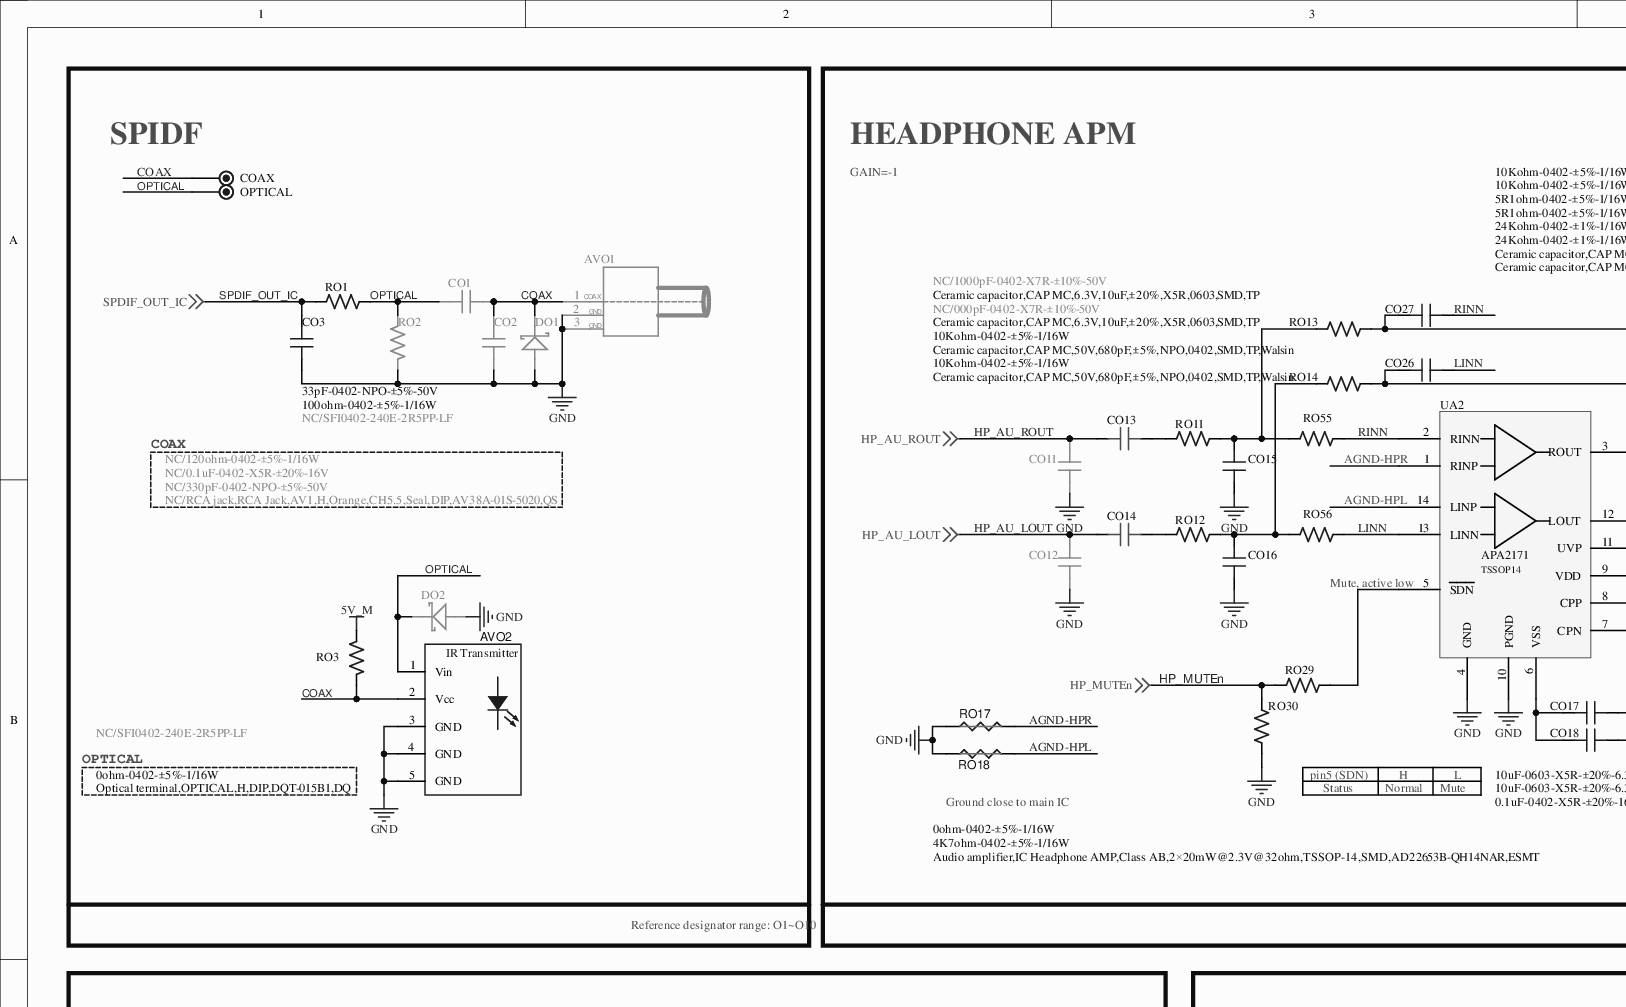
[diagram p0: MISC86290-14.SchDoc, top left]
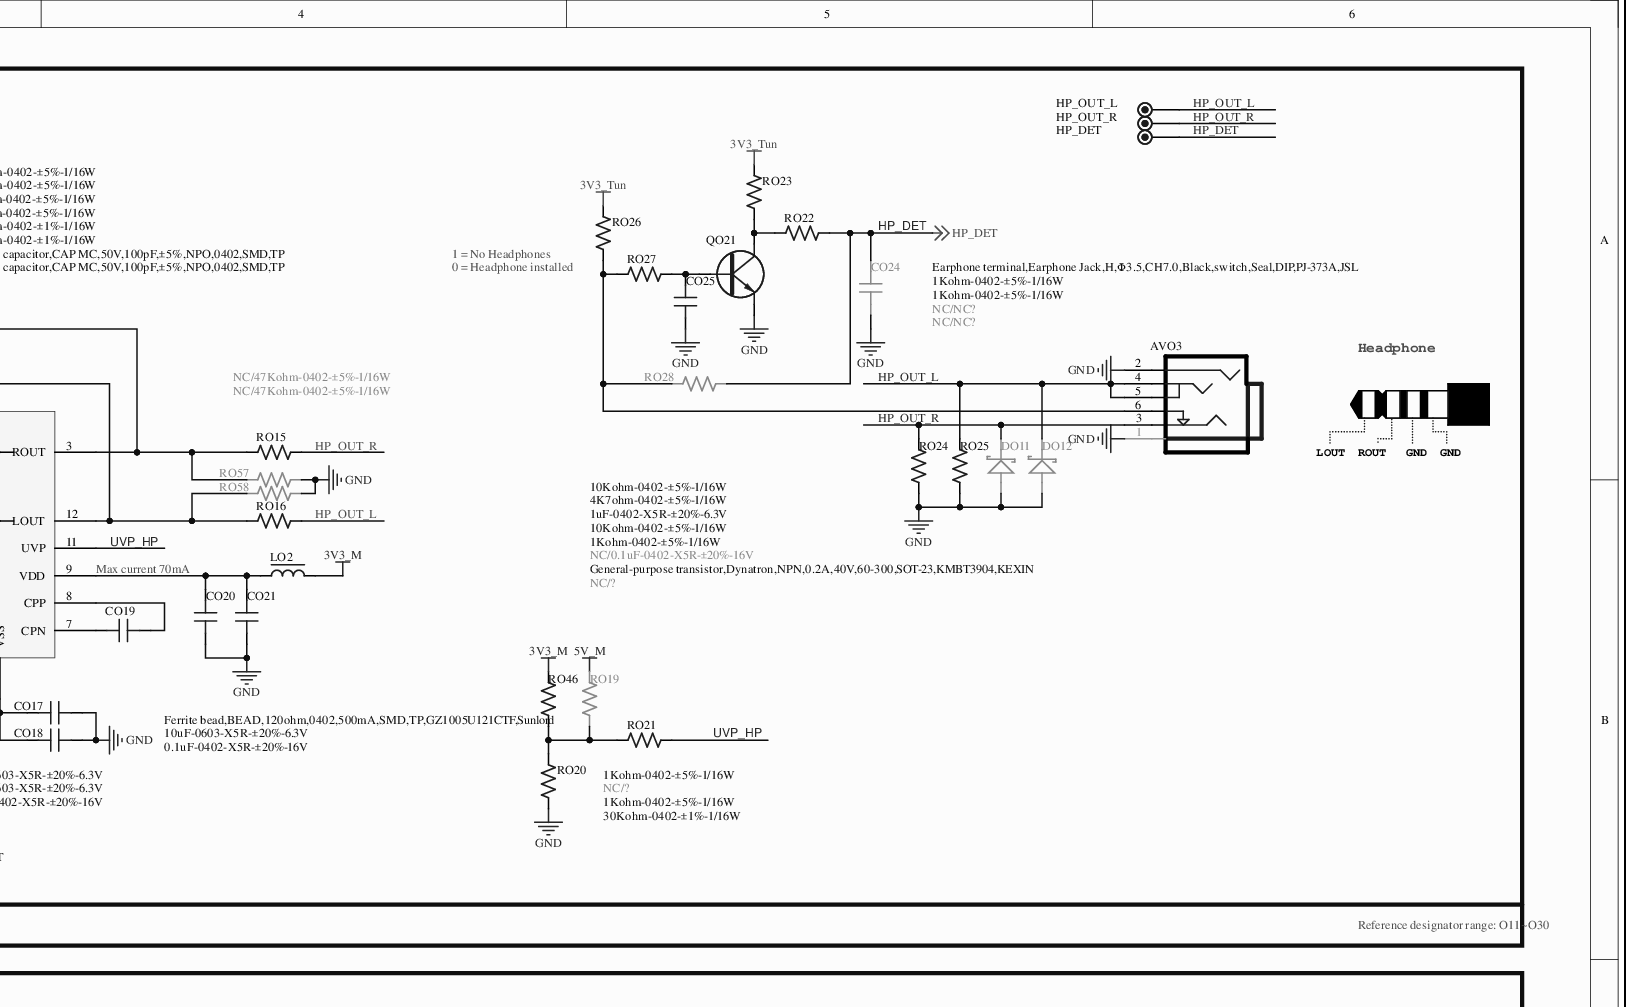
[diagram p1: MISC86290-14.SchDoc, top right]
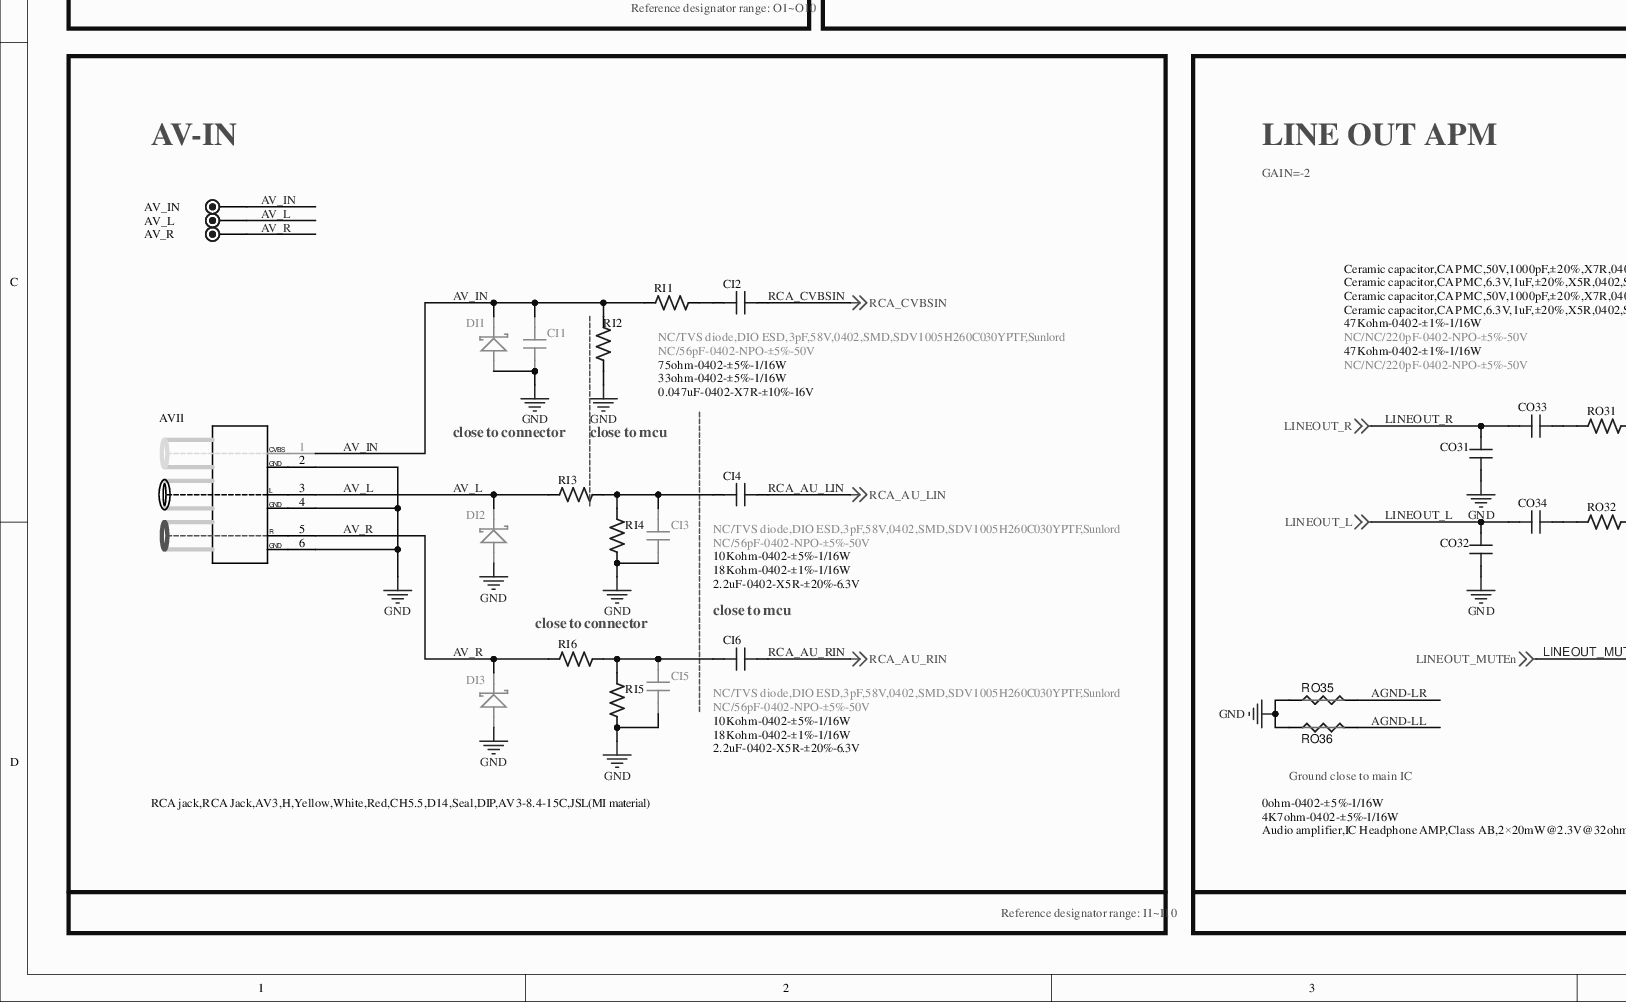
[diagram p2: MISC86290-14.SchDoc, bottom left]
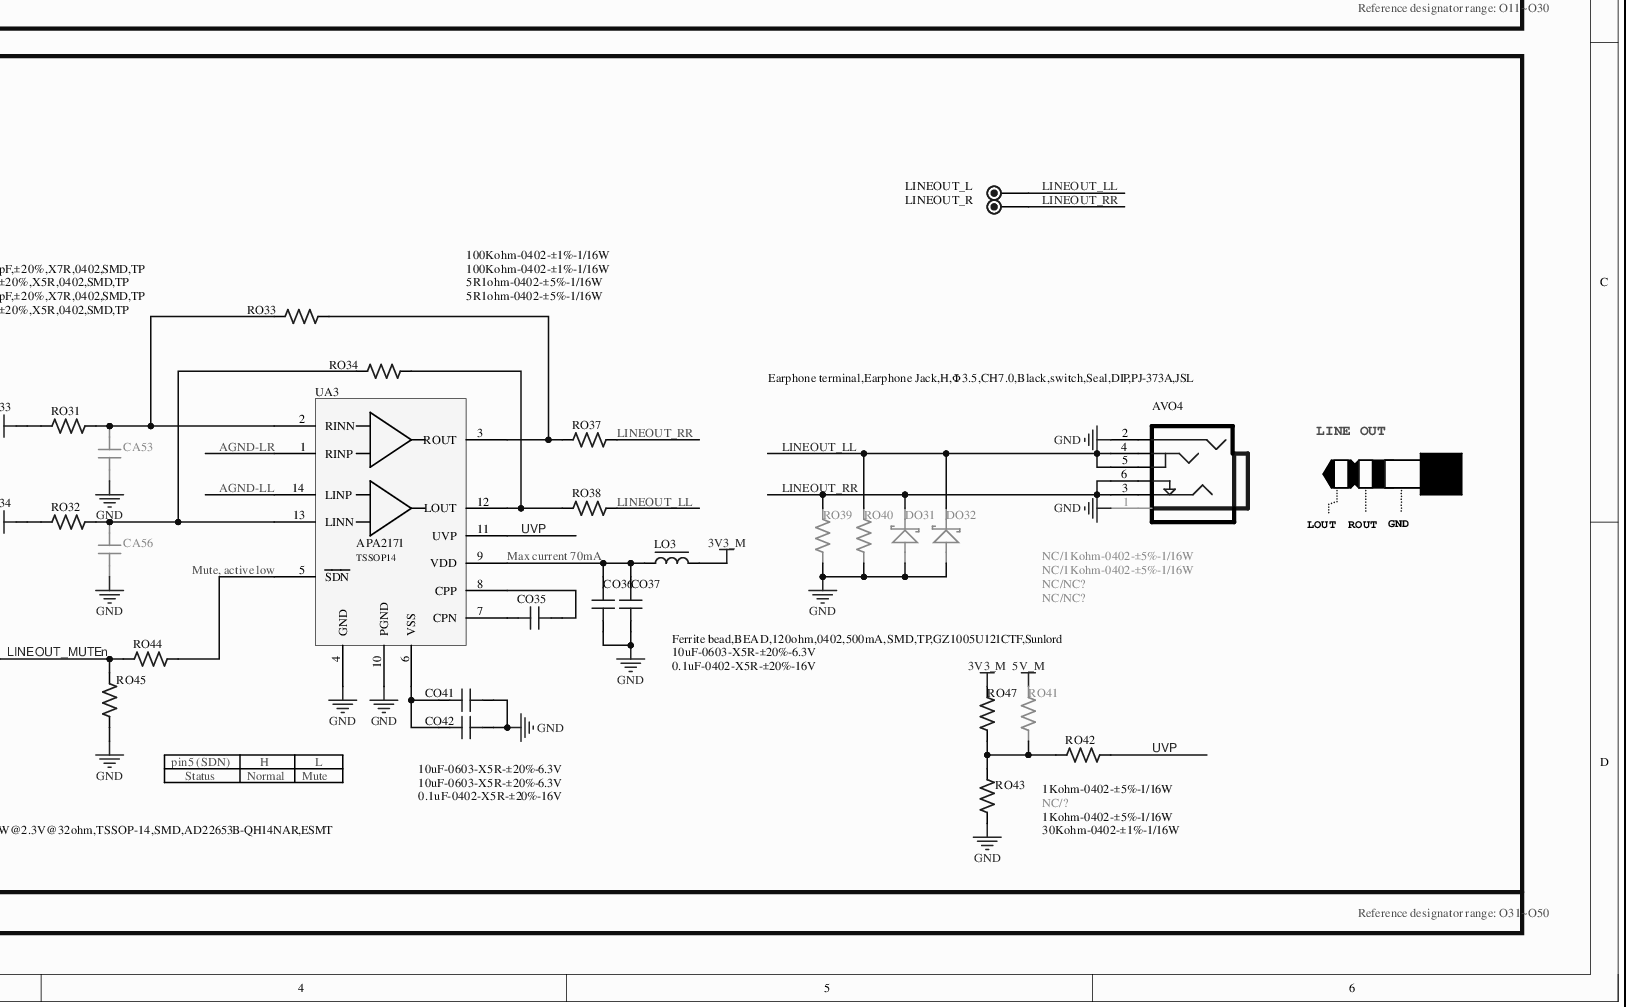
[diagram p3: MISC86290-14.SchDoc, bottom right]
# Altium project MISC86290.PrjPcb (part 10 of 13)

## Sheet MISC86290-14.SchDoc
size 584 x 355 mm

### Parts
(Parts that share a designator on the sheet are numbered #1, #2 ... from top to bottom, then left to right.)
AV_IN  TEST  [TP]  (value not drawn)
AV_L  TEST  [TP]  (value not drawn)
AV_R  TEST  [TP]  (value not drawn)
AVI1  RCA jack,RCA Jack,AV3,H,Yellow,White,Red,CH5.5,D14,Seal,DIP,AV3-8.4-15C,JSL(MI material)  [AV3-H14-15]
AVO1  NC/RCA jack,RCA Jack,AV1,H,Orange,CH5.5,Seal,DIP,AV38A-01S-5020,QS  [AV1-H-4]
AVO2  Optical terminal,OPTICAL,H,DIP,DQT-015B1,DQ  [OPTICAL-HD-6]
AVO3  Earphone terminal,Earphone Jack,H,Φ3.5,CH7.0,Black,switch,Seal,DIP,PJ-373A,JSL  [PHONE-HD-42]
AVO4  Earphone terminal,Earphone Jack,H,Φ3.5,CH7.0,Black,switch,Seal,DIP,PJ-373A,JSL  [PHONE-HD-42]
CA53  NC/NC/220pF-0402-NPO-±5%-50V  [C0402]
CA56  NC/NC/220pF-0402-NPO-±5%-50V  [C0402]
CI1  NC/56pF-0402-NPO-±5%-50V  [C0402]
CI2  0.047uF-0402-X7R-±10%-16V  [C0402]
CI3  NC/56pF-0402-NPO-±5%-50V  [C0402]
CI4  2.2uF-0402-X5R-±20%-6.3V  [C0402]
CI5  NC/56pF-0402-NPO-±5%-50V  [C0402]
CI6  2.2uF-0402-X5R-±20%-6.3V  [C0402]
CO1  NC/0.1uF-0402-X5R-±20%-16V  [C0402]
CO2  NC/330pF-0402-NPO-±5%-50V  [C0402]
CO3  33pF-0402-NPO-±5%-50V  [C0402]
CO11  NC/1000pF-0402-X7R-±10%-50V  [C0402]
CO12  NC/000pF-0402-X7R-±10%-50V  [C0402]
CO13  Ceramic capacitor,CAP MC,6.3V,10uF,±20%,X5R,0603,SMD,TP  [C0603]
CO14  Ceramic capacitor,CAP MC,6.3V,10uF,±20%,X5R,0603,SMD,TP  [C0603]
CO15  Ceramic capacitor,CAP MC,50V,680pF,±5%,NPO,0402,SMD,TP,Walsin  [C0402]
CO16  Ceramic capacitor,CAP MC,50V,680pF,±5%,NPO,0402,SMD,TP,Walsin  [C0402]
CO17  10uF-0603-X5R-±20%-6.3V  [C0603]
CO18  0.1uF-0402-X5R-±20%-16V  [C0402]
CO19  10uF-0603-X5R-±20%-6.3V  [C0603]
CO20  10uF-0603-X5R-±20%-6.3V  [C0603]
CO21  0.1uF-0402-X5R-±20%-16V  [C0402]
CO24  NC/0.1uF-0402-X5R-±20%-16V  [C0402]
CO25  1uF-0402-X5R-±20%-6.3V  [C0402]
CO26  Ceramic capacitor,CAP MC,50V,100pF,±5%,NPO,0402,SMD,TP  [C0402]
CO27  Ceramic capacitor,CAP MC,50V,100pF,±5%,NPO,0402,SMD,TP  [C0402]
CO31  Ceramic capacitor,CAP MC,50V,1000pF,±20%,X7R,0402,SMD,TP  [C0402]
CO32  Ceramic capacitor,CAP MC,50V,1000pF,±20%,X7R,0402,SMD,TP  [C0402]
CO33  Ceramic capacitor,CAP MC,6.3V,1uF,±20%,X5R,0402,SMD,TP  [C0402]
CO34  Ceramic capacitor,CAP MC,6.3V,1uF,±20%,X5R,0402,SMD,TP  [C0402]
CO35  10uF-0603-X5R-±20%-6.3V  [C0603]
CO36  10uF-0603-X5R-±20%-6.3V  [C0603]
CO37  0.1uF-0402-X5R-±20%-16V  [C0402]
CO41  10uF-0603-X5R-±20%-6.3V  [C0603]
CO42  0.1uF-0402-X5R-±20%-16V  [C0402]
COAX#2  TEST  [TP]  (value not drawn)
DI1  NC/TVS diode,DIO ESD,3pF,58V,0402,SMD,SDV1005H260C030YPTF,Sunlord  [DIODE-S0402]
DI2  NC/TVS diode,DIO ESD,3pF,58V,0402,SMD,SDV1005H260C030YPTF,Sunlord  [DIODE-S0402]
DI3  NC/TVS diode,DIO ESD,3pF,58V,0402,SMD,SDV1005H260C030YPTF,Sunlord  [DIODE-S0402]
DO1  NC/SFI0402-240E-2R5PP-LF  [DIODE-S0402]
DO2  NC/SFI0402-240E-2R5PP-LF  [DIODE-S0402]
DO11  NC/NC?  [DIODE-S0402]
DO12  NC/NC?  [DIODE-S0402]
DO31  NC/NC?  [DIODE-S0402]
DO32  NC/NC?  [DIODE-S0402]
HP_DET  TEST  [TP]  (value not drawn)
HP_OUT_L  TEST  [TP]  (value not drawn)
HP_OUT_R  TEST  [TP]  (value not drawn)
LINEOUT_L  TEST  [TP]  (value not drawn)
LINEOUT_R  TEST  [TP]  (value not drawn)
LO2  Ferrite bead,BEAD,120ohm,0402,500mA,SMD,TP,GZ1005U121CTF,Sunlord  [L0402]
LO3  Ferrite bead,BEAD,120ohm,0402,500mA,SMD,TP,GZ1005U121CTF,Sunlord  [L0402]
OPTICAL#2  TEST  [TP]  (value not drawn)
QO21  General-purpose transistor,Dynatron,NPN,0.2A,40V,60-300,SOT-23,KMBT3904,KEXIN  [SOT-23]
RI1  33ohm-0402-±5%-1/16W  [R0402]
RI2  75ohm-0402-±5%-1/16W  [R0402]
RI3  10Kohm-0402-±5%-1/16W  [R0402]
RI4  18Kohm-0402-±1%-1/16W  [R0402]
RI5  18Kohm-0402-±1%-1/16W  [R0402]
RI6  10Kohm-0402-±5%-1/16W  [R0402]
RO1  100ohm-0402-±5%-1/16W  [R0402]
RO2  NC/120ohm-0402-±5%-1/16W  [R0402]
RO3  0ohm-0402-±5%-1/16W  [R0402]
RO11  10Kohm-0402-±5%-1/16W  [R0402]
RO12  10Kohm-0402-±5%-1/16W  [R0402]
RO13  10Kohm-0402-±5%-1/16W  [R0402]
RO14  10Kohm-0402-±5%-1/16W  [R0402]
RO15  5R1ohm-0402-±5%-1/16W  [R0402]
RO16  5R1ohm-0402-±5%-1/16W  [R0402]
RO17  NC/SHORT  [GND]  (value not drawn)
RO18  NC/SHORT  [GND]  (value not drawn)
RO19  NC/?  [R0402]
RO20  1Kohm-0402-±5%-1/16W  [R0402]
RO21  30Kohm-0402-±1%-1/16W  [R0402]
RO22  1Kohm-0402-±5%-1/16W  [R0402]
RO23  10Kohm-0402-±5%-1/16W  [R0402]
RO24  1Kohm-0402-±5%-1/16W  [R0402]
RO25  1Kohm-0402-±5%-1/16W  [R0402]
RO26  10Kohm-0402-±5%-1/16W  [R0402]
RO27  4K7ohm-0402-±5%-1/16W  [R0402]
RO28  NC/?  [R0402]
RO29  0ohm-0402-±5%-1/16W  [R0402]
RO30  4K7ohm-0402-±5%-1/16W  [R0402]
RO31  47Kohm-0402-±1%-1/16W  [R0402]
RO32  47Kohm-0402-±1%-1/16W  [R0402]
RO33  100Kohm-0402-±1%-1/16W  [R0402]
RO34  100Kohm-0402-±1%-1/16W  [R0402]
RO35  NC/SHORT  [GND]  (value not drawn)
RO36  NC/SHORT  [GND]  (value not drawn)
RO37  5R1ohm-0402-±5%-1/16W  [R0402]
RO38  5R1ohm-0402-±5%-1/16W  [R0402]
RO39  NC/1Kohm-0402-±5%-1/16W  [R0402]
RO40  NC/1Kohm-0402-±5%-1/16W  [R0402]
RO41  NC/?  [R0402]
RO42  30Kohm-0402-±1%-1/16W  [R0402]
RO43  1Kohm-0402-±5%-1/16W  [R0402]
RO44  0ohm-0402-±5%-1/16W  [R0402]
RO45  4K7ohm-0402-±5%-1/16W  [R0402]
RO46  1Kohm-0402-±5%-1/16W  [R0402]
RO47  1Kohm-0402-±5%-1/16W  [R0402]
RO55  24Kohm-0402-±1%-1/16W  [R0402]
RO56  24Kohm-0402-±1%-1/16W  [R0402]
RO57  NC/47Kohm-0402-±5%-1/16W  [R0402]
RO58  NC/47Kohm-0402-±5%-1/16W  [R0402]
UA2  Audio amplifier,IC Headphone AMP,Class AB,2×20mW@2.3V@32ohm,TSSOP-14,SMD,AD22653B-QH14NAR,ESMT  [SSOP14/0.65-1]
UA3  Audio amplifier,IC Headphone AMP,Class AB,2×20mW@2.3V@32ohm,TSSOP-14,SMD,AD22653B-QH14NAR,ESMT  [SSOP14/0.65-1]

### Blocks framed on the sheet
SPIDF: AVO1 AVO2 CO1-CO3 COAX#2 DO1 DO2 OPTICAL#2 RO1-RO3
HEADPHONE APM: AVO3 CO11-CO21 CO24-CO27 DO11 DO12 HP_DET HP_OUT_L HP_OUT_R LO2 QO21 RO11-RO30 RO46 RO55-RO58 UA2
AV-IN: AV_IN AV_L AV_R AVI1 CI1-CI6 DI1-DI3 RI1-RI6
LINE OUT APM: AVO4 CA53 CA56 CO31-CO37 CO41 CO42 DO31 DO32 LINEOUT_L LINEOUT_R LO3 RO31-RO45 RO47 UA3

### Nets
3V3_M: LO2.2 LO3.2 RO46.2 RO47.2
3V3_Tun: RO23.1 RO26.1
5V_M: RO3.1 RO19.2 RO41.2
GND: AVI1.2(GND) AVI1.4 AVI1.6 AVO1.2(GND) AVO1.3(GND) AVO2.3(GND) AVO2.4(GND) AVO2.5(GND) AVO3.1 AVO3.2 AVO4.1 AVO4.2 CA53.1 CA56.1 CI1.1 CI3.1 CI5.1 CO2.1 CO3.1 CO11.1 CO12.1 CO15.1 CO16.1 CO17.2 CO18.2 CO20.1 CO21.1 CO24.1 CO25.1 CO31.1 CO32.1 CO36.1 CO37.1 CO41.2 CO42.2 DI1.A DI2.A DI3.A DO1.A DO2.A DO11.A DO12.A DO31.A DO32.A QO21.E RI2.1 RI4.1 RI5.1 RO2.1 RO17.JP_2K RO18.JP_2K RO20.1 RO24.1 RO25.1 RO30.1 RO35.JP_2K RO36.JP_2K RO39.1 RO40.1 RO43.1 RO45.1 RO57.1 RO58.1 UA2.4(GND) UA2.10(PGND) UA3.4(GND) UA3.10(PGND)
AGND-HPL: RO18.JP_1K UA2.14(LINP)
AGND-HPR: RO17.JP_1K UA2.1(RINP)
AGND-LL: RO36.JP_1K UA3.14(LINP)
AGND-LR: RO35.JP_1K UA3.1(RINP)
AV_IN: AV_IN.1 AVI1.1(R) CI1.2 DI1.K RI1.1 RI2.2
AV_L: AV_L.1 AVI1.3 DI2.K RI3.1
AV_R: AV_R.1 AVI1.5 DI3.K RI6.1
COAX: AVO1.1(CVBS) AVO2.2(Vcc) CO1.2 CO2.2 COAX#2.1 DO1.K RO3.2
HP_AU_LOUT: CO12.2 CO14.2 ; off-sheet HP_AU_LOUT
HP_AU_ROUT: CO11.2 CO13.2 ; off-sheet HP_AU_ROUT
HP_DET: CO24.2 HP_DET.1 RO22.2 RO28.2 ; off-sheet HP_DET
HP_MUTEn: RO29.1 RO30.2 ; off-sheet HP_MUTEn
HP_OUT_L: AVO3.4 AVO3.5 DO12.K HP_OUT_L.1 RO16.2 RO25.2
HP_OUT_R: AVO3.3 DO11.K HP_OUT_R.1 RO15.2 RO24.2
LINEOUT_L: CO32.2 CO34.1 ; off-sheet LINEOUT_L
LINEOUT_LL: AVO4.4 AVO4.5 DO32.K LINEOUT_L.1 RO38.2 RO40.2
LINEOUT_MUTEn: RO44.1 RO45.2 ; off-sheet LINEOUT_MUTEn
LINEOUT_R: CO31.2 CO33.1 ; off-sheet LINEOUT_R
LINEOUT_RR: AVO4.3 AVO4.6 DO31.K LINEOUT_R.1 RO37.2 RO39.2
LINN: CO26.2 RO56.2 UA2.13(LINN)
OPTICAL: AVO2.1(Vin) CO1.1 DO2.K OPTICAL#2.1 RO1.2 RO2.2
RCA_AU_LIN: CI4.2 ; off-sheet RCA_AU_LIN
RCA_AU_RIN: CI6.2 ; off-sheet RCA_AU_RIN
RCA_CVBSIN: CI2.2 ; off-sheet RCA_CVBSIN
RINN: CO27.2 RO55.2 UA2.2(RINN)
SPDIF_OUT_IC: CO3.2 RO1.1 ; off-sheet SPDIF_OUT_IC
UVP: RO42.2 UA3.11(UVP)
UVP_HP: RO21.2 UA2.11(UVP)
NetAVO3_6: AVO3.6 RO26.2 RO27.2 RO28.1
NetCA53_2: CA53.2 RO31.2 RO33.1 UA3.2(RINN)
NetCA56_2: CA56.2 RO32.2 RO34.1 UA3.13(LINN)
NetCI2_1: CI2.1 RI1.2
NetCI3_2: CI3.2 CI4.1 RI3.2 RI4.2
NetCI5_2: CI5.2 CI6.1 RI5.2 RI6.2
NetCO13_1: CO13.1 RO11.1
NetCO14_1: CO14.1 RO12.1
NetCO15_2: CO15.2 RO11.2 RO13.1 RO55.1
NetCO16_2: CO16.2 RO12.2 RO14.1 RO56.1
NetCO17_1: CO17.1 CO18.1 UA2.6(VSS)
NetCO19_1: CO19.1 UA2.7(CPN)
NetCO19_2: CO19.2 UA2.8(CPP)
NetCO20_2: CO20.2 CO21.2 LO2.1 UA2.9(VDD)
NetCO25_2: CO25.2 QO21.B RO27.1
NetCO26_1: CO26.1 RO14.2 RO16.1 RO58.2 UA2.12(LOUT)
NetCO27_1: CO27.1 RO13.2 RO15.1 RO57.2 UA2.3(ROUT)
NetCO33_2: CO33.2 RO31.1
NetCO34_2: CO34.2 RO32.1
NetCO35_1: CO35.1 UA3.7(CPN)
NetCO35_2: CO35.2 UA3.8(CPP)
NetCO36_2: CO36.2 CO37.2 LO3.1 UA3.9(VDD)
NetCO41_1: CO41.1 CO42.1 UA3.6(VSS)
NetQO21_C: QO21.C RO22.1 RO23.2
NetRO19_1: RO19.1 RO20.2 RO21.1 RO46.1
NetRO29_2: RO29.2 UA2.5(~{SDN})
NetRO33_2: RO33.2 RO37.1 UA3.3(ROUT)
NetRO34_2: RO34.2 RO38.1 UA3.12(LOUT)
NetRO41_1: RO41.1 RO42.1 RO43.2 RO47.1
NetRO44_2: RO44.2 UA3.5(~{SDN})

### Notes on the sheet
- GAIN=-1
- (near RO26) 0 = Headphone installed
- 1 = No Headphones
- Headphone
- COAX
- LOUT
- ROUT
- GND
- Max current 70mA
- (near UA2) Mute, active low
- OPTICAL
- pin5 (SDN)
- H
- L
- (near RO18) Ground close to main IC
- Status
- Normal
- Mute
- Reference designator range: O1~O10
- Reference designator range: O11~O30
- GAIN=-2
- close to connector
- close to mcu
- LINE OUT
- (near CI6) close to mcu
- (near UA3) Mute, active low
- (near RO36) Ground close to main IC
- Reference designator range: I1~I10
- Reference designator range: O31~O50

### Library data of the parts
AVI1 = RCA端子,RCA Jack,AV3,H,Yellow、White、Red,CH5.5,D14,Seal,DIP,RC075-F03L3BY-A,YUQIU-DLMI-AV: CN-AV-D14-#-#
AVO1 = RCA端子,RCA Jack,AV1,H,Orange,CH5.5,Seal,DIP,AV38A-01S-5020,QS-DLMI
AVO2 = XXX.XXX.0002291: Optical terminal,OPTICAL,H,DIP,DQT-015B1,DQ-DLMI
AVO3 AVO4 = XXX.XXX.0002138: Earphone terminal,Earphone Jack,H,Φ3.5,CH7.0,Black,switch,Seal,DIP,PJ7724-F05L3BY-D,YUQIU-DLMI
CA53 CA56 CO15 CO16 = 220pF-0402-NPO-±5%-50V-D
CI1 CI3 CI5 = 56pF-0402-NPO-±5%-50V-D
CI2 = 0.047uF-0402-X7R-±10%-16V-D
CI4 CI6 = 1uF-0402-X5R-±20%-16V-D
CO1 CO21 CO24 CO25 CO37 = 0.1uF-0402-X5R-±20%-16V-D
CO2 = 330pF-0402-NPO-±5%-50V-D
CO3 = 33pF-0402-NPO-±5%-50V-D
CO11 CO12 CO31 CO32 = 1000pF-0402-X7R-±10%-50V-D
CO13 CO14 = 004.003.0000383-D: Ceramic capacitor,CAP MC,6.3V,10uF,±20%,X5R,0603,SMD,TP-D
CO17 CO19 CO35 CO41 = 10uF-0603-X5R-±20%-6.3V-D
CO18 CO42 = 0.1uF-0402-X7R-±10%-16V-D
CO20 CO36 = 10uF-0603-X5R-±20%-6.3
CO26 CO27 = 004.003.0000501-D: Ceramic capacitor,CAP MC,50V,100pF,±5%,NPO,0402,SMD,TP-D
CO33 CO34 = 1uF-0402-X5R-±20%-6.3V-D
DI1-DI3 DO1 DO2 DO11 DO12 DO31 DO32 = AVLC18S02003-D
LO2 LO3 = 004.004.0000326-D: Ferrite bead,BEAD,120ohm,0402,500mA,SMD,TP,FCM1005KF-121T06,Tai-tech-D
QO21 = LMBT3904LT1G-D-NPN: Q-NPN-#-#-#
RI1 = 33ohm-0402-±5%-1/16W-D
RI2 RO2 = 75ohm-0402-±5%-1/16W-D
RI3 RI6 = 10Kohm-0402-±5%-1/16W-D
RI4 RI5 RO19 RO21 RO41 RO42 = 12Kohm-0402-±5%-1/16W-D
RO1 = 200ohm-0402-±5%-1/16W-D
RO3 = 0ohm-0402-±5%-1/16W-D
RO11 RO12 RO31 RO32 = 33Kohm-0402-±5%-1/16W-D
RO13 RO14 RO33 RO34 RO55 RO56 = 100Kohm-0402-±5%-1/16W-D
RO15 RO16 RO37 RO38 = 5R1ohm-0402-±5%-1/16W-D
RO17 RO18 RO35 RO36 = GND: Manufacturer: Panasonic; Part Number: ERJ3GEYJ473V; Right: 20; Bottom: 30; CLASS: Discrete; Comments: Digikey
RO20 RO22 RO23 RO26-RO30 RO43-RO47 = 4K7ohm-0402-±5%-1/16W-D
RO24 RO25 RO39 RO40 = 1Kohm-0402-±5%-1/16W-D
RO57 RO58 = 47Kohm-0402-±5%-1/16W-D
UA2 UA3 = APA2171-D